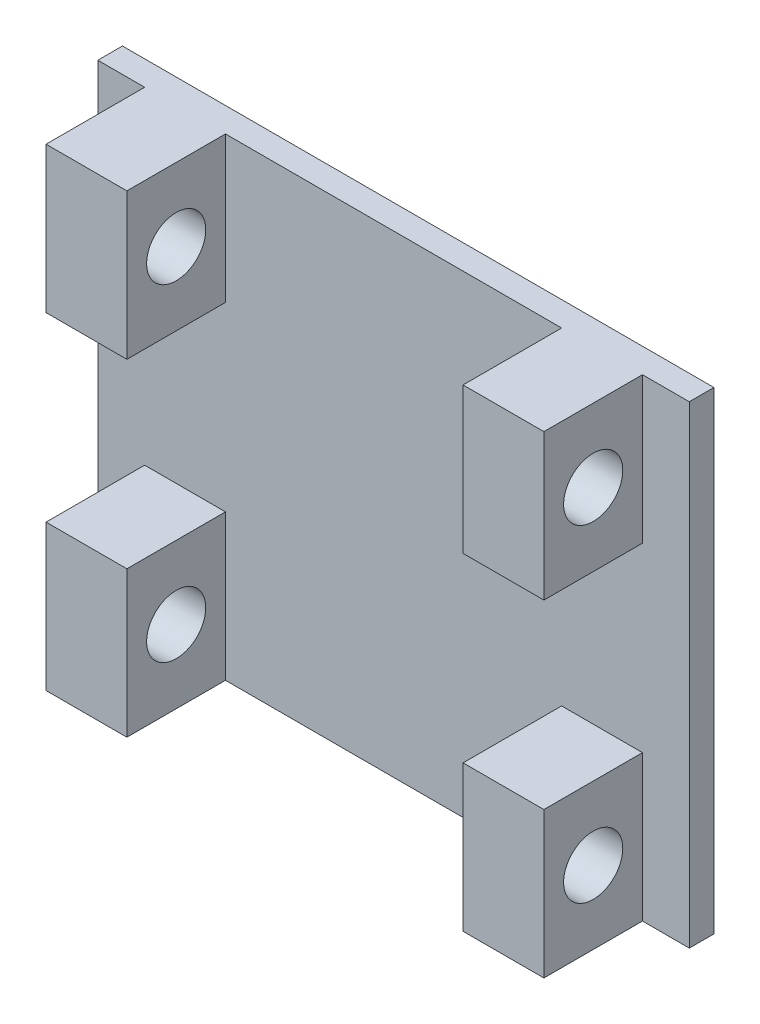
from build123d import *

# Parameters (mm, degrees)
SKETCH1_W           = 600
SKETCH1_H           = 480
BOSS_EXTRUDE1_DEPTH = 25
SKETCH2_W           = 82
SKETCH2_H           = 148
BOSS_EXTRUDE2_DEPTH = 100
SKETCH4_R           = 30
CUT_EXTRUDE1_DEPTH  = 743.483164792
SKETCH5_R           = 65
SKETCH5_R_2         = 40
BOSS_EXTRUDE3_DEPTH = 20
SKETCH6_R           = 60
SKETCH6_R_2         = 40
BOSS_EXTRUDE4_DEPTH = 77
SKETCH7_R           = 40
BOSS_EXTRUDE5_DEPTH = 12.5


with BuildPart() as part:
    # Sketch1 → Boss-Extrude1 (new body)
    with BuildSketch(Plane.XY):
        with Locations((300, 240)):
            Rectangle(SKETCH1_W, SKETCH1_H)
    extrude(amount=BOSS_EXTRUDE1_DEPTH)

    # Sketch2 → Boss-Extrude2 (add)
    with BuildSketch(Plane.XY.offset(25)):
        with Locations((88.5, 406)):
            Rectangle(SKETCH2_W, SKETCH2_H)
        with Locations((88.5, 74)):
            Rectangle(SKETCH2_W, SKETCH2_H)
        with Locations((511.5, 74)):
            Rectangle(SKETCH2_W, SKETCH2_H)
        with Locations((511.5, 406)):
            Rectangle(SKETCH2_W, SKETCH2_H)
    extrude(amount=BOSS_EXTRUDE2_DEPTH)

    # Sketch4 → Cut-Extrude1 (cut, through all)
    with BuildSketch(Plane.ZY.offset(-47.5)):
        with Locations(Location((75, 406, 0), (0, 0, 180))):
            Circle(SKETCH4_R)
        with Locations(Location((75, 74, 0), (0, 0, 180))):
            Circle(SKETCH4_R)
    extrude(amount=-CUT_EXTRUDE1_DEPTH, mode=Mode.SUBTRACT)

    # Sketch5 → Boss-Extrude3 (add)
    with BuildSketch(Plane(origin=(0, 0, 0), x_dir=(-1, 0, 0), z_dir=(0, 0, -1))):
        with Locations((-300, 240)):
            Circle(SKETCH5_R)
        with Locations((-300, 240)):
            Circle(SKETCH5_R_2, mode=Mode.SUBTRACT)
    extrude(amount=BOSS_EXTRUDE3_DEPTH)

    # Sketch6 → Boss-Extrude4 (add)
    with BuildSketch(Plane(origin=(0, 0, -20), x_dir=(-1, 0, 0), z_dir=(0, 0, -1))):
        with Locations((-300, 240)):
            Circle(SKETCH6_R)
        with Locations((-300, 240)):
            Circle(SKETCH6_R_2, mode=Mode.SUBTRACT)
    extrude(amount=BOSS_EXTRUDE4_DEPTH)

    # Sketch7 → Boss-Extrude5 (add)
    with BuildSketch(Plane(origin=(0, 0, 0), x_dir=(-1, 0, 0), z_dir=(0, 0, -1))):
        with Locations((-300, 240)):
            Circle(SKETCH7_R)
    extrude(amount=BOSS_EXTRUDE5_DEPTH)


solid = part.part
